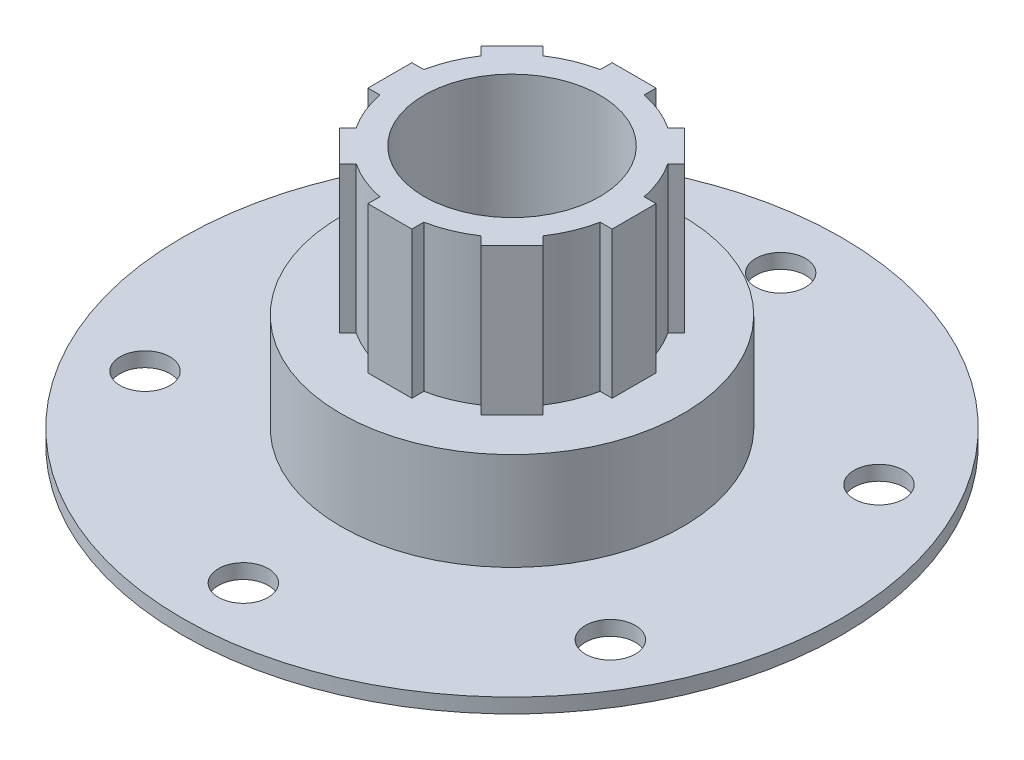
SolidWorks part; units mm, degrees
ref_plane "前视基准面" through (0, 0, 0) normal (0, 0, 1) x (1, 0, 0)
ref_plane "上视基准面" through (0, 0, 0) normal (0, 1, 0) x (1, 0, 0)
ref_plane "右视基准面" through (0, 0, 0) normal (1, 0, 0) x (0, 0, -1)
sketch "草图1" plane through (0, 0, 0) normal (0, 1, 0) x (1, 0, 0)
  circle A0 centre (0, 0) radius 67.5
  circle A1 centre (0, 0) radius 18
extrude "凸台-拉伸1" add sketch "草图1" along normal blind 53
sketch "草图2" plane through (0, 53, 0) normal (0, 1, 0) x (1, 0, 0)
  circle A0 centre (0, 0) radius 35
extrude "切除-拉伸1" cut sketch "草图2" against normal blind 50 flip side to cut
sketch "草图3" plane through (0, 53, 0) normal (0, 1, 0) x (1, 0, 0)
  circle A0 centre (0, 0) radius 23
extrude "切除-拉伸2" cut sketch "草图3" against normal blind 30 flip side to cut
sketch "草图4" plane through (0, 53, 0) normal (0, 1, 0) x (1, 0, 0)
  line L0 (0, 0) -> (0, 50000) construction
  line L1 (0, 25) -> (4.5, 25)
  line L2 (4.5, 25) -> (4.5, 18.6591)
  line L3 (4.5, 18.6591) -> (-4.5, 18.6591)
  line L4 (-4.5, 18.6591) -> (-4.5, 25)
  line L5 (-4.5, 25) -> (0, 25)
  line L6 (10.012, 16.376) -> (14.4957, 20.8597)
  line L7 (14.4957, 20.8597) -> (17.6777, 17.6777)
  line L8 (17.6777, 17.6777) -> (20.8597, 14.4957)
  line L9 (20.8597, 14.4957) -> (16.376, 10.012)
  line L10 (16.376, 10.012) -> (10.012, 16.376)
  line L11 (18.6591, 4.5) -> (25, 4.5)
  line L12 (25, 4.5) -> (25, 0)
  line L13 (25, 0) -> (25, -4.5)
  line L14 (25, -4.5) -> (18.6591, -4.5)
  line L15 (18.6591, -4.5) -> (18.6591, 4.5)
  line L16 (16.376, -10.012) -> (20.8597, -14.4957)
  line L17 (20.8597, -14.4957) -> (17.6777, -17.6777)
  line L18 (17.6777, -17.6777) -> (14.4957, -20.8597)
  line L19 (14.4957, -20.8597) -> (10.012, -16.376)
  line L20 (10.012, -16.376) -> (16.376, -10.012)
  line L21 (4.5, -18.6591) -> (4.5, -25)
  line L22 (4.5, -25) -> (0, -25)
  line L23 (0, -25) -> (-4.5, -25)
  line L24 (-4.5, -25) -> (-4.5, -18.6591)
  line L25 (-4.5, -18.6591) -> (4.5, -18.6591)
  line L26 (-10.012, -16.376) -> (-14.4957, -20.8597)
  line L27 (-14.4957, -20.8597) -> (-17.6777, -17.6777)
  line L28 (-17.6777, -17.6777) -> (-20.8597, -14.4957)
  line L29 (-20.8597, -14.4957) -> (-16.376, -10.012)
  line L30 (-16.376, -10.012) -> (-10.012, -16.376)
  line L31 (-18.6591, -4.5) -> (-25, -4.5)
  line L32 (-25, -4.5) -> (-25, 0)
  line L33 (-25, 0) -> (-25, 4.5)
  line L34 (-25, 4.5) -> (-18.6591, 4.5)
  line L35 (-18.6591, 4.5) -> (-18.6591, -4.5)
  line L36 (-16.376, 10.012) -> (-20.8597, 14.4957)
  line L37 (-20.8597, 14.4957) -> (-17.6777, 17.6777)
  line L38 (-17.6777, 17.6777) -> (-14.4957, 20.8597)
  line L39 (-14.4957, 20.8597) -> (-10.012, 16.376)
  line L40 (-10.012, 16.376) -> (-16.376, 10.012)
  point P45 (0, 0)
  dimension "D1" = 25
  dimension "D2" = 9
  dimension "D3" = 8
extrude "凸台-拉伸2" add sketch "草图4" against normal up to surface (30 mm away) up to face at (0, 23, 35)
sketch "草图5" plane through (0, 3, 0) normal (0, 1, 0) x (1, 0, 0)
  line L0 (0, 0) -> (0, 50000) construction
  line L1 (0, 0) -> (43301.2702, 25000) construction
  line L2 (0, 0) -> (43301.2702, -25000) construction
  circle A0 centre (0, 0) radius 55 construction
  dimension "D1" = 60
  dimension "D2" = 60
hole_wizard "M12 螺纹孔的螺纹孔钻头1" positions "草图7" profile "草图6" hole size "M12" standard "Iso"
sketch "草图7" plane through (0, 3, 0) normal (0, 1, 0) x (1, 0, 0)
  line L0 (0, -200000) -> (0, 250000) construction
  line L1 (-173205.0808, 100000) -> (216506.3509, -125000) construction
  line L2 (-173205.0808, -100000) -> (216506.3509, 125000) construction
  circle A0 centre (0, 0) radius 55 construction
  point P0 (0, 55)
  point P6 (-47.6314, 27.5)
  point P10 (-47.6314, -27.5)
  point P14 (0, -55)
  point P16 (47.6314, -27.5)
  point P18 (47.6314, 27.5)
sketch "草图6" plane through (0, 3, -55) normal (1, 0, 0) x (0, 0, 1)
  line L0 (0, 0) -> (0, 8.0644)
  line L1 (0, 8.0644) -> (5.1, 5)
  line L2 (5.1, 5) -> (5.1, 0)
  line L5 (5.1, 0) -> (0, 0)
  line L10 (0, 8.0644) -> (-5.1, 5) construction
  line L11 (0, -6.35) -> (0, 107.95) construction
  dimension "孔直径" = 10.2
  dimension "孔深度" = 5
  dimension "导头角度" = 118
